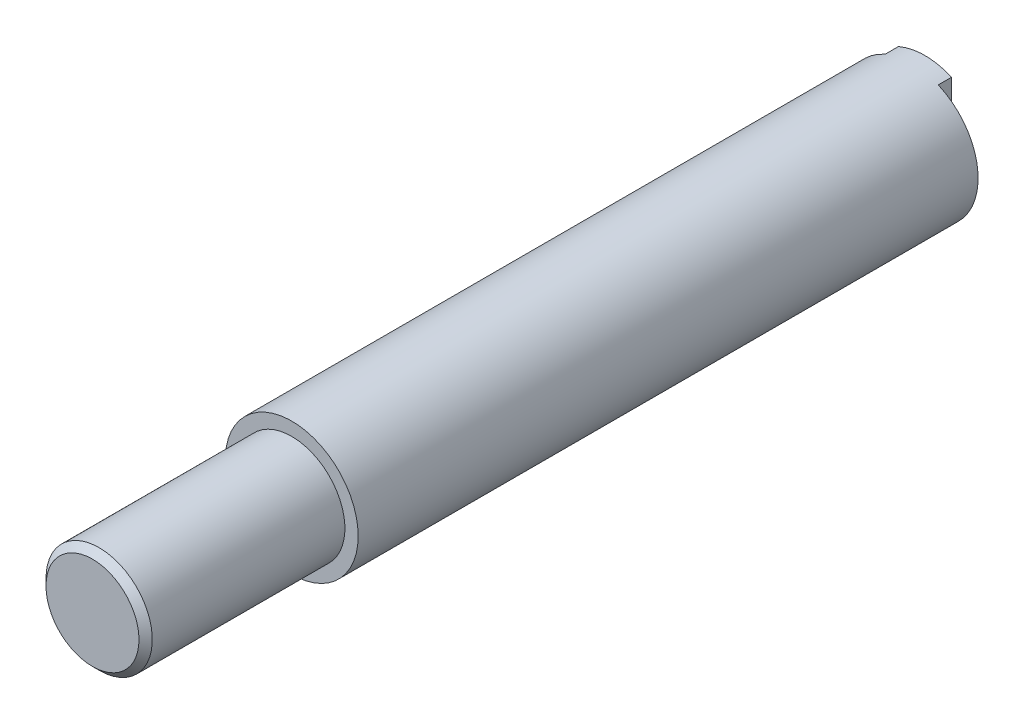
from build123d import *
from build123d.topology import SkipClean

# Parameters (mm, degrees)
SKETCH1_R              = 15
BOSS_EXTRUDE1_DEPTH    = 140
SKETCH2_R              = 12
BOSS_EXTRUDE2_DEPTH    = 45
BOSS_EXTRUDE3_START    = 3
BOSS_EXTRUDE3_DEPTH    = 3
M10_TAPPED_HOLE1_D     = 8.5
M10_TAPPED_HOLE1_DEPTH = 24.5
M10_TAPPED_HOLE1_TIP   = 2.553657631
CHAMFER1_SIZE          = 1.5


with BuildPart() as part:
    # Sketch1 → Boss-Extrude1 (new body)
    with BuildSketch(Plane.XY):
        Circle(SKETCH1_R)
    extrude(amount=BOSS_EXTRUDE1_DEPTH)

    # Sketch2 → Boss-Extrude2 (add)
    with BuildSketch(Plane.XY.offset(140)):
        with Locations(Location((0, 0, 0), (0, 0, 180))):
            Circle(SKETCH2_R)
    extrude(amount=BOSS_EXTRUDE2_DEPTH)

    # Sketch3 → Boss-Extrude3 (add)
    with SkipClean():  # the faces are left unmerged after this step: merging them gives an invalid solid
        with BuildSketch(Plane(origin=(0, 0, 0), x_dir=(-1, 0, 0), z_dir=(0, 0, -1)).offset(BOSS_EXTRUDE3_START)):
            with BuildLine():
                Line((-6, 13.747727085), (-6, -13.747727085))
                ThreePointArc((-6, -13.747727085), (0, -15), (6, -13.747727085))
                Line((6, -13.747727085), (6, 13.747727085))
                ThreePointArc((6, 13.747727085), (0, 15), (-6, 13.747727085))
            make_face()
        extrude(amount=-BOSS_EXTRUDE3_DEPTH)

    # M10 Tapped Hole1
    with Locations(Plane(origin=(0, 0, -3), x_dir=(-1, 0, 0), z_dir=(0, 0, -1))):
        with Locations((0, 0)):
            Hole(M10_TAPPED_HOLE1_D / 2, depth=M10_TAPPED_HOLE1_DEPTH)
            with Locations((0, 0, -(M10_TAPPED_HOLE1_DEPTH + M10_TAPPED_HOLE1_TIP / 2))):  # 118° drill point
                Cone(0, M10_TAPPED_HOLE1_D / 2, M10_TAPPED_HOLE1_TIP, mode=Mode.SUBTRACT)

    # Chamfer1
    chamfer1_edges = [part.edges().sort_by_distance(p)[0] for p in [
        (12, 0, 185),
    ]]
    chamfer(chamfer1_edges, length=CHAMFER1_SIZE)


solid = part.part
